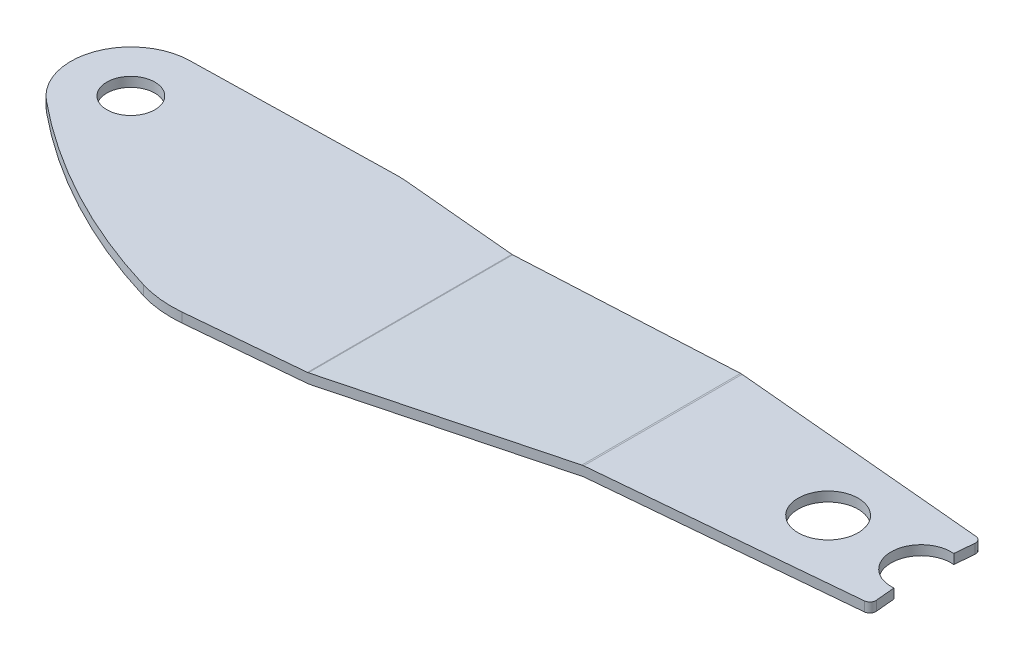
from build123d import *

# Parameters (mm, degrees)
BOSS_EXTRUDE1_DEPTH = 600
SKETCH4_OUTSIDE_W   = 1933.152
SKETCH4_OUTSIDE_H   = 942.352
SKETCH4_OUTSIDE_R   = 40
SKETCH4_OUTSIDE_R_2 = 50
CUT_EXTRUDE1_DEPTH  = 1121.500446229


with BuildPart() as part:
    # Sketch1 → Boss-Extrude1 (new body)
    with BuildSketch(Plane.XY):
        with BuildLine():
            Line((-1.216429586, 8), (-647.3, 8))
            Line((-647.3, 8), (-647.3, -8))
            Line((-647.3, -8), (-0.810953057, -8))
            ThreePointArc((-0.810953057, -8), (0.537559565, -7.954486055), (1.879934575, -7.818151371))
            Line((1.879934575, -7.818151371), (419.67098577, 48.909075685))
            ThreePointArc((419.67098577, 48.909075685), (420.342173275, 48.977243027), (421.016429586, 49))
            Line((421.016429586, 49), (943.5, 49))
            Line((943.5, 49), (943.5, 65))
            Line((943.5, 65), (420.610953057, 65))
            ThreePointArc((420.610953057, 65), (419.262440435, 64.954486055), (417.920065425, 64.818151371))
            Line((417.920065425, 64.818151371), (0.12901423, 8.090924315))
            ThreePointArc((0.12901423, 8.090924315), (-0.542173275, 8.022756973), (-1.216429586, 8))
        make_face()
    extrude(amount=BOSS_EXTRUDE1_DEPTH)

    # Sketch4 outside → Cut-Extrude1 (cut, through all)
    # profile 1 of 3: a face of its own
    with BuildSketch(Plane(origin=(0, 65, 0), x_dir=(1, 0, 0), z_dir=(0, 1, 0))):
        with Locations((148.1, -300)):
            Rectangle(SKETCH4_OUTSIDE_W, SKETCH4_OUTSIDE_H)
        with BuildLine():
            Line((849.441033389, -393.022786976), (-192.741176471, -487.726520609))
            ThreePointArc((-192.741176471, -487.726520609), (-228.733049722, -487.54676651), (-264.034655196, -480.529366519))
            ThreePointArc((-264.034655196, -480.529366519), (-446.549262984, -405.356942265), (-610.742483166, -295.798456192))
            ThreePointArc((-610.742483166, -295.798456192), (-641.798915546, -185.789833988), (-549.379294824, -118.521619672))
            Line((-549.379294824, -118.521619672), (-213.719470744, -111.540753082))
            ThreePointArc((-213.719470744, -111.540753082), (-203.220116273, -111.614875507), (-192.741176471, -112.273479391))
            Line((-192.741176471, -112.273479391), (849.441033389, -206.977213024))
            ThreePointArc((849.441033389, -206.977213024), (856.218024477, -210.53404245), (858.495022624, -217.84115701))
            Line((858.495022624, -217.84115701), (855.553845389, -250.207806915))
            ThreePointArc((855.553845389, -250.207806915), (801, -300), (855.553845389, -349.792193085))
            Line((855.553845389, -349.792193085), (858.495022624, -382.15884299))
            ThreePointArc((858.495022624, -382.15884299), (856.218024477, -389.46595755), (849.441033389, -393.022786976))
        make_face(mode=Mode.SUBTRACT)
    # profile 2 of 3: a face of its own
    with BuildSketch(Plane(origin=(0, 65, 0), x_dir=(1, 0, 0), z_dir=(0, 1, 0))):
        with Locations(Location((-547.3, -218.5, 0), (0, 0, 180))):
            Circle(SKETCH4_OUTSIDE_R)
    # profile 3 of 3: a face of its own
    with BuildSketch(Plane(origin=(0, 65, 0), x_dir=(1, 0, 0), z_dir=(0, 1, 0))):
        with Locations(Location((696, -300, 0), (0, 0, 180))):
            Circle(SKETCH4_OUTSIDE_R_2)
    extrude(amount=-CUT_EXTRUDE1_DEPTH, mode=Mode.SUBTRACT)


solid = part.part
